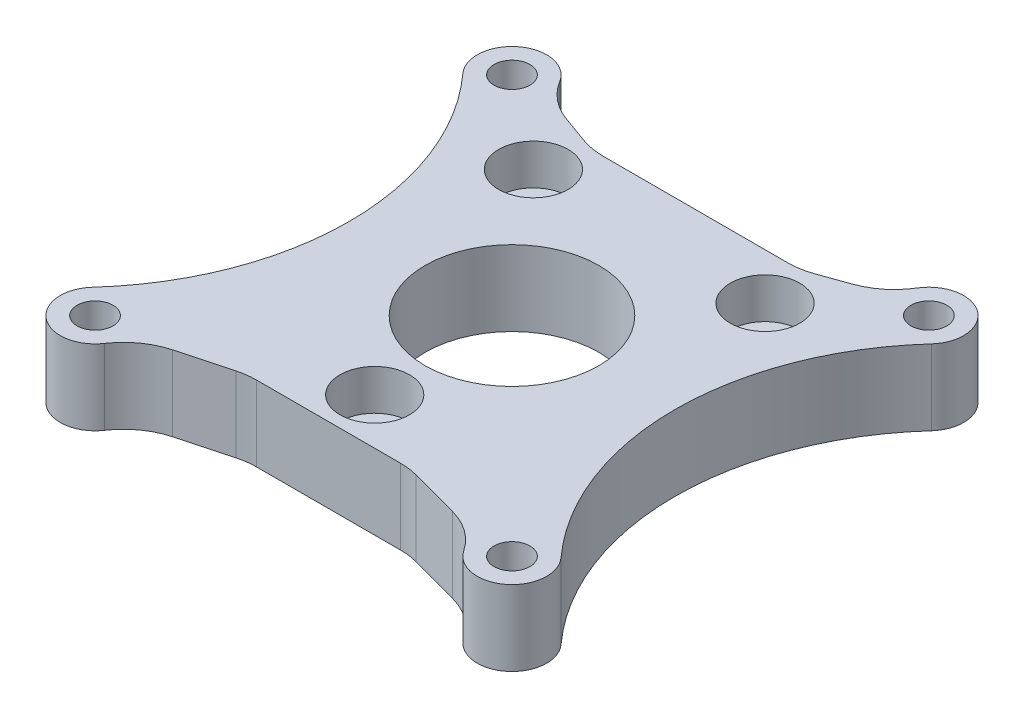
from build123d import *

# Parameters (mm, degrees)
SKETCH_1_R           = 1.55
EXTRUDE_1_DEPTH      = 6.5
FILLET_1_R           = 6
SKETCH_9_R           = 7.5
SKETCH_9_R_2         = 1.55
CUT_EXTRUDE_11_DEPTH = 31.401480227
SKETCH_10_R          = 3
CUT_EXTRUDE_12_DEPTH = 3.5


with BuildPart() as part:
    # 草图1 → 凸台-拉伸1 (new body)
    with BuildSketch(Plane(origin=(0, 0, 0), x_dir=(1, 0, 0), z_dir=(0, 1, 0))):
        with BuildLine():
            Line((-15, 18), (-9, 15.85))
            Line((-9, 15.85), (9, 15.85))
            Line((9, 15.85), (15, 18))
            ThreePointArc((15, 18), (19.079157226, 20.799181966), (20.223613121, 15.986161702))
            ThreePointArc((20.223613121, 15.986161702), (14.060533289, 0), (20.223613121, -15.986161702))
            ThreePointArc((20.223613121, -15.986161702), (19.079157226, -20.799181966), (15, -18))
            Line((15, -18), (7, -15.85))
            Line((7, -15.85), (-7, -15.85))
            Line((-7, -15.85), (-15, -18))
            ThreePointArc((-15, -18), (-19.079157226, -20.799181966), (-20.223613121, -15.986161702))
            ThreePointArc((-20.223613121, -15.986161702), (-14.060533289, 0), (-20.223613121, 15.986161702))
            ThreePointArc((-20.223613121, 15.986161702), (-19.079157226, 20.799181966), (-15, 18))
        make_face()
        with Locations(Location((18, 18, 0), (0, 0, 90))):
            Circle(SKETCH_1_R, mode=Mode.SUBTRACT)
        with Locations(Location((18, -18, 0), (0, 0, 90))):
            Circle(SKETCH_1_R, mode=Mode.SUBTRACT)
        with Locations(Location((-18, -18, 0), (0, 0, 90))):
            Circle(SKETCH_1_R, mode=Mode.SUBTRACT)
        with Locations(Location((-18, 18, 0), (0, 0, 90))):
            Circle(SKETCH_1_R, mode=Mode.SUBTRACT)
    extrude(amount=EXTRUDE_1_DEPTH)

    # 圆角1
    fillet_1_edges = [part.edges().sort_by_distance(p)[0] for p in [
        (15, 3.25, 18),
        (7, 3.25, 15.85),
        (-7, 3.25, 15.85),
        (-15, 3.25, 18),
        (-15, 3.25, -18),
        (-9, 3.25, -15.85),
        (9, 3.25, -15.85),
        (15, 3.25, -18),
    ]]
    fillet(fillet_1_edges, radius=FILLET_1_R)

    # 草图9 → 切除-拉伸11 (cut, through all)
    with BuildSketch(Plane(origin=(0, 6.5, 0), x_dir=(1, 0, 0), z_dir=(0, 1, 0))):
        with Locations(Location((0, 0, 0), (0, 0, 270))):
            Circle(SKETCH_9_R)
        with Locations(Location((10, 11.85, 0), (0, 0, 270))):
            Circle(SKETCH_9_R_2)
        with Locations(Location((0, -11.85, 0), (0, 0, 270))):
            Circle(SKETCH_9_R_2)
        with Locations(Location((-10, 11.85, 0), (0, 0, 270))):
            Circle(SKETCH_9_R_2)
    extrude(amount=-CUT_EXTRUDE_11_DEPTH, mode=Mode.SUBTRACT)

    # 草图10 → 切除-拉伸12 (cut)
    with BuildSketch(Plane(origin=(0, 6.5, 0), x_dir=(1, 0, 0), z_dir=(0, 1, 0))):
        with Locations(Location((-10, 11.85, 0), (0, 0, 270))):
            Circle(SKETCH_10_R)
        with Locations(Location((10, 11.85, 0), (0, 0, 270))):
            Circle(SKETCH_10_R)
        with Locations(Location((0, -11.85, 0), (0, 0, 270))):
            Circle(SKETCH_10_R)
    extrude(amount=-CUT_EXTRUDE_12_DEPTH, mode=Mode.SUBTRACT)


solid = part.part
